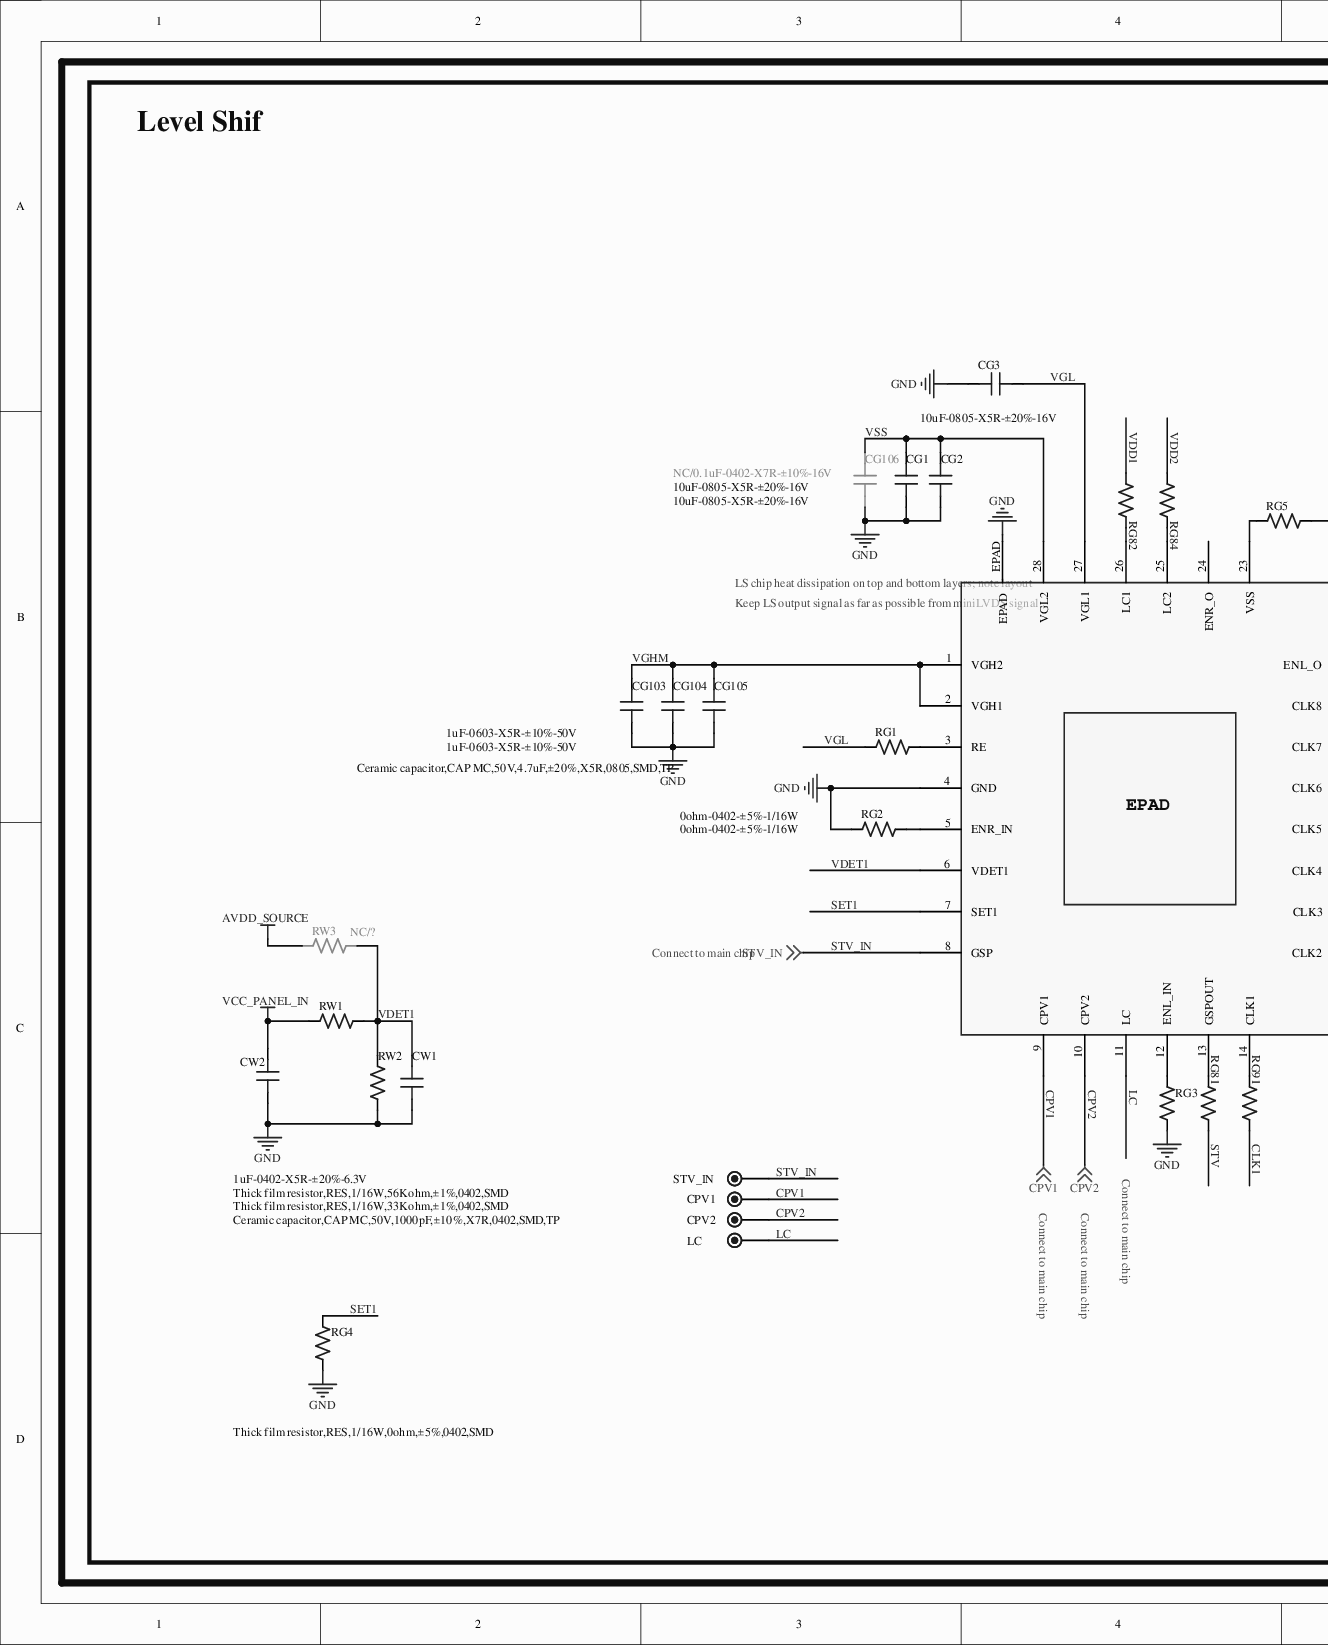
[diagram p0: MISC84395-19.SchDoc, left]
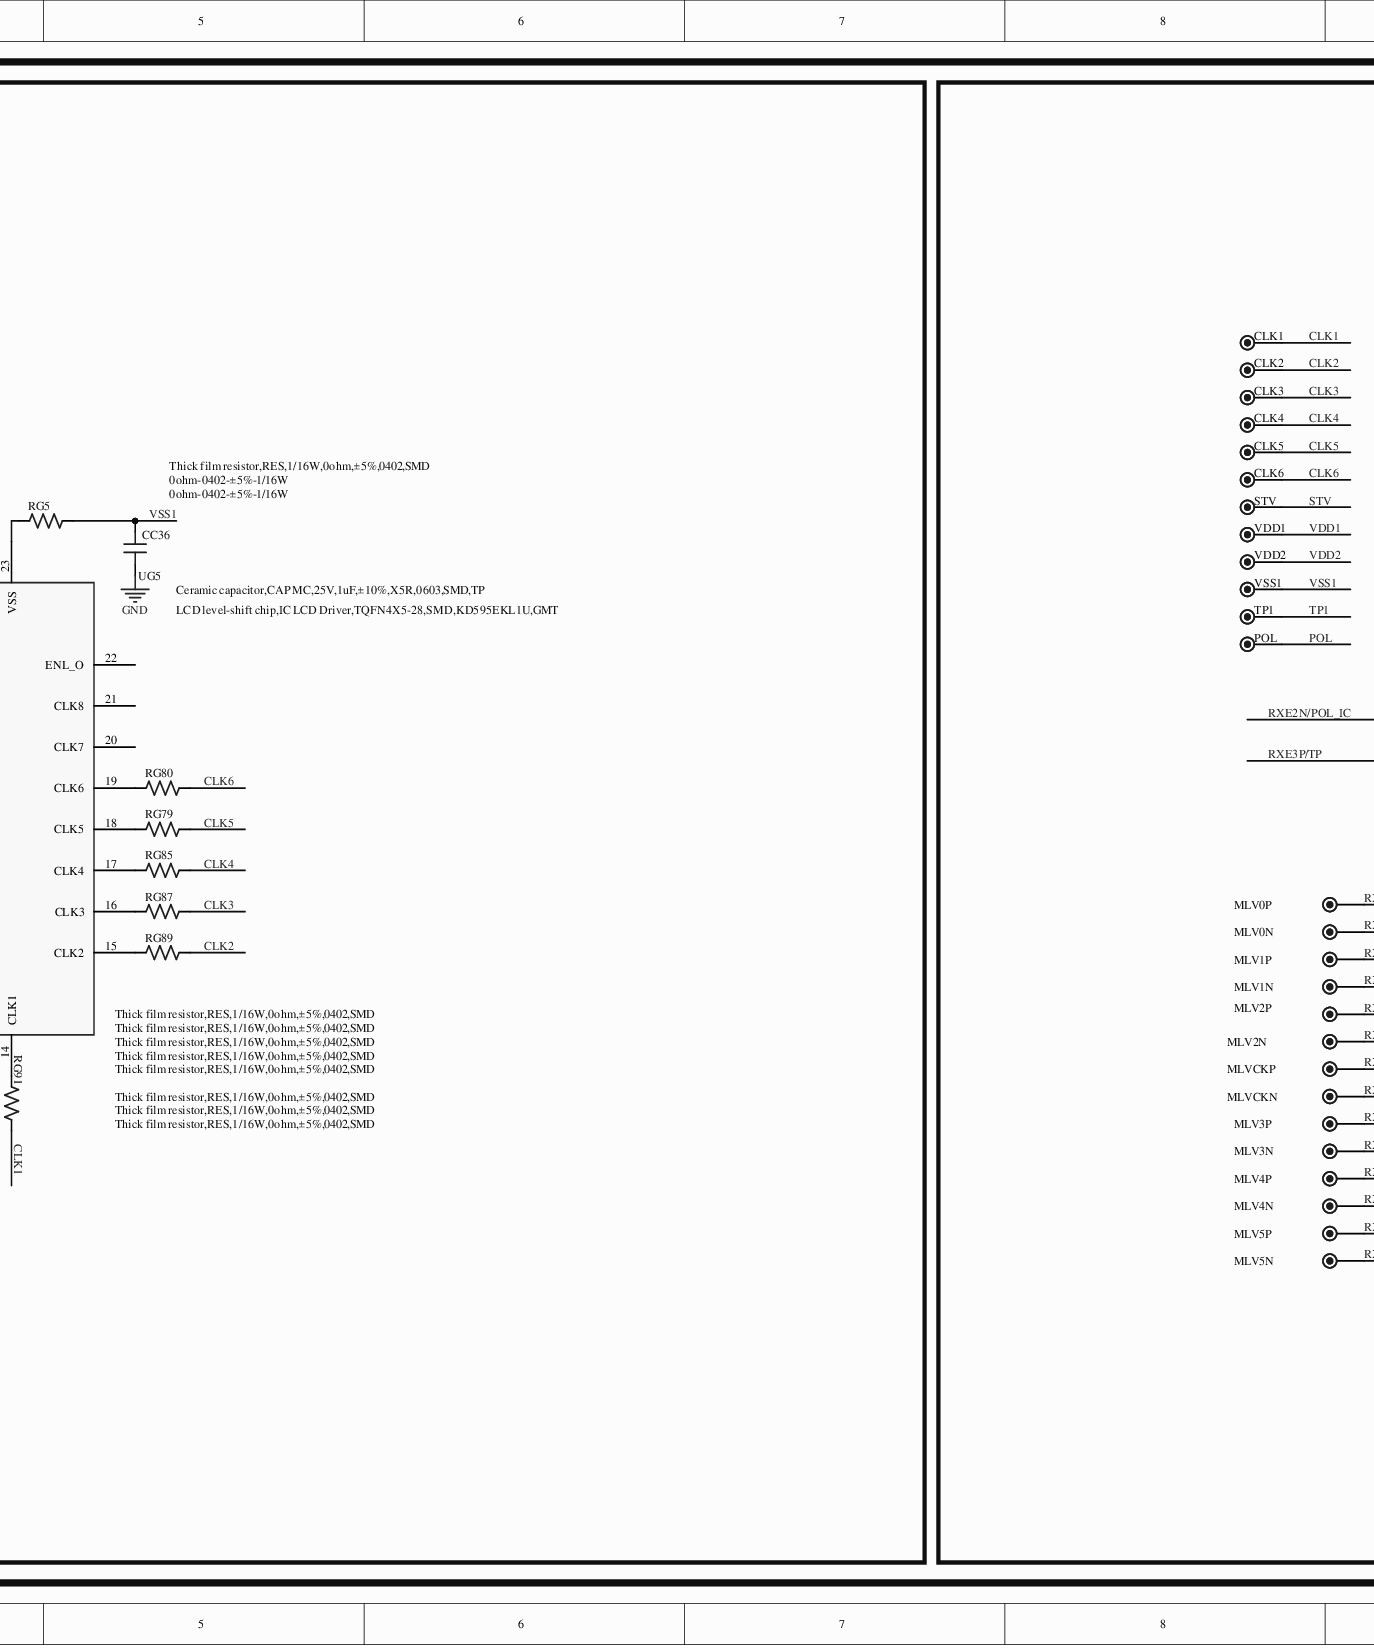
[diagram p1: MISC84395-19.SchDoc, middle]
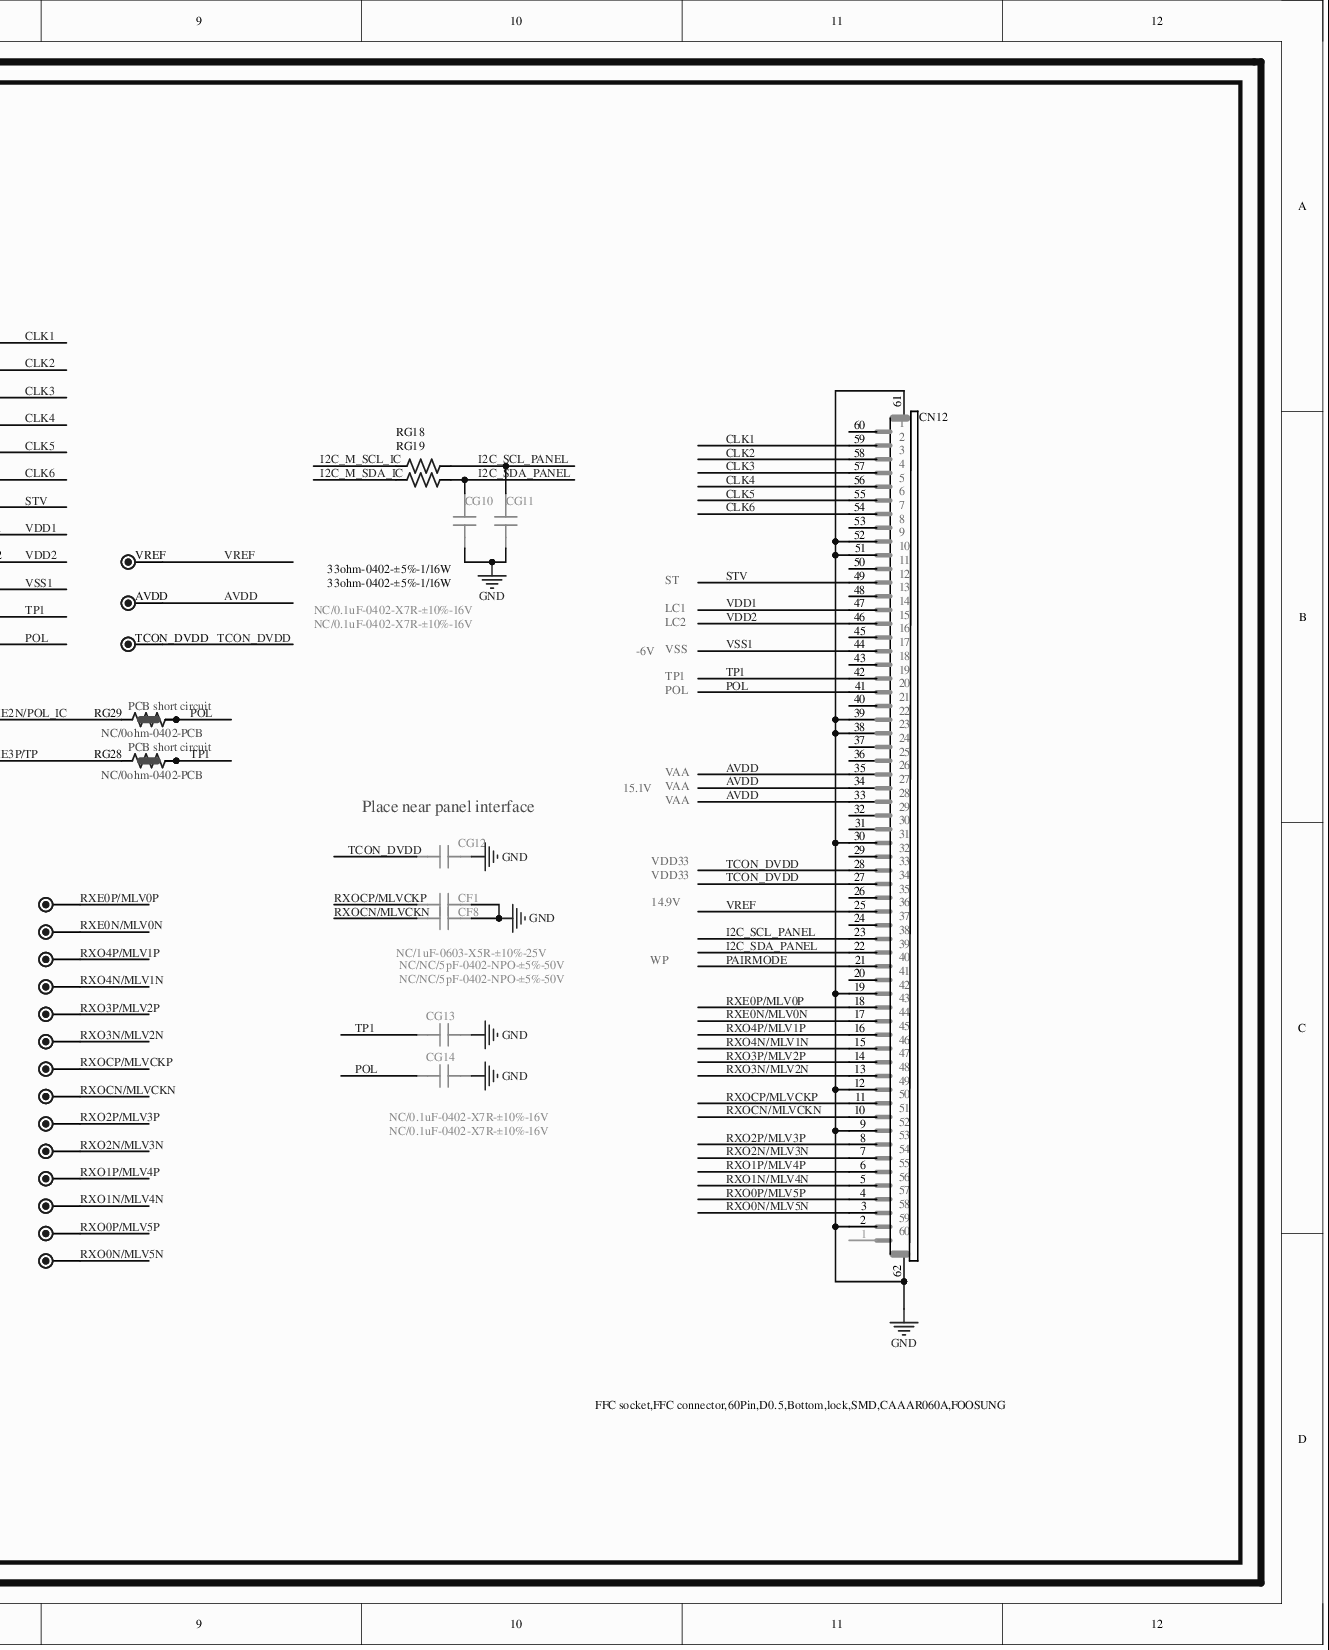
[diagram p2: MISC84395-19.SchDoc, right]
# Altium project MISC84395-37.PrjPCB (part 13 of 13)

## Sheet MISC84395-19.SchDoc
size 711 x 304 mm

### Parts
AVDD  TEST  [TP]  (value not drawn)
CC36  Ceramic capacitor,CAP MC,25V,1uF,±10%,X5R,0603,SMD,TP  [C0603]
CF1  NC/NC/5pF-0402-NPO-±5%-50V  [C0402]
CF8  NC/NC/5pF-0402-NPO-±5%-50V  [C0402]
CG1  10uF-0805-X5R-±20%-16V  [C0805]
CG2  10uF-0805-X5R-±20%-16V  [C0805]
CG3  10uF-0805-X5R-±20%-16V  [C0805]
CG10  NC/0.1uF-0402-X7R-±10%-16V  [C0402]
CG11  NC/0.1uF-0402-X7R-±10%-16V  [C0402]
CG12  NC/1uF-0603-X5R-±10%-25V  [C0603]
CG13  NC/0.1uF-0402-X7R-±10%-16V  [C0402]
CG14  NC/0.1uF-0402-X7R-±10%-16V  [C0402]
CG103  1uF-0603-X5R-±10%-50V  [C0603]
CG104  Ceramic capacitor,CAP MC,50V,4.7uF,±20%,X5R,0805,SMD,TP  [C0805]
CG105  1uF-0603-X5R-±10%-50V  [C0603]
CG106  NC/0.1uF-0402-X7R-±10%-16V  [C0402]
CLK1  TEST  [TP]  (value not drawn)
CLK2  TEST  [TP]  (value not drawn)
CLK3  TEST  [TP]  (value not drawn)
CLK4  TEST  [TP]  (value not drawn)
CLK5  TEST  [TP]  (value not drawn)
CLK6  TEST  [TP]  (value not drawn)
CN12  FFC socket,FFC connector,60Pin,D0.5,Bottom,lock,SMD,CAAAR060A,FOOSUNG  [FFC60H/0.5S-13]
CPV1  TEST  [TP]  (value not drawn)
CPV2  TEST  [TP]  (value not drawn)
CW1  Ceramic capacitor,CAP MC,50V,1000pF,±10%,X7R,0402,SMD,TP  [C0402]
CW2  1uF-0402-X5R-±20%-6.3V  [C0402]
LC  TEST  [TP]  (value not drawn)
MLV0N  TEST  [TP]  (value not drawn)
MLV0P  TEST  [TP]  (value not drawn)
MLV1N  TEST  [TP]  (value not drawn)
MLV1P  TEST  [TP]  (value not drawn)
MLV2N  TEST  [TP]  (value not drawn)
MLV2P  TEST  [TP]  (value not drawn)
MLV3N  TEST  [TP]  (value not drawn)
MLV3P  TEST  [TP]  (value not drawn)
MLV4N  TEST  [TP]  (value not drawn)
MLV4P  TEST  [TP]  (value not drawn)
MLV5N  TEST  [TP]  (value not drawn)
MLV5P  TEST  [TP]  (value not drawn)
MLVCKN  TEST  [TP]  (value not drawn)
MLVCKP  TEST  [TP]  (value not drawn)
POL  TEST  [TP]  (value not drawn)
RG1  0ohm-0402-±5%-1/16W  [R0402]
RG2  0ohm-0402-±5%-1/16W  [R0402]
RG3  Thick film resistor,RES,1/16W,0ohm,±5%,0402,SMD  [R0402]
RG4  Thick film resistor,RES,1/16W,0ohm,±5%,0402,SMD  [R0402]
RG5  0ohm-0402-±5%-1/16W  [R0402]
RG18  33ohm-0402-±5%-1/16W  [R0402]
RG19  33ohm-0402-±5%-1/16W  [R0402]
RG28  NC/0ohm-0402-PCB  [R0402SC]
RG29  NC/0ohm-0402-PCB  [R0402SC]
RG79  Thick film resistor,RES,1/16W,0ohm,±5%,0402,SMD  [R0402]
RG80  Thick film resistor,RES,1/16W,0ohm,±5%,0402,SMD  [R0402]
RG81  Thick film resistor,RES,1/16W,0ohm,±5%,0402,SMD  [R0402]
RG82  Thick film resistor,RES,1/16W,0ohm,±5%,0402,SMD  [R0402]
RG84  0ohm-0402-±5%-1/16W  [R0402]
RG85  Thick film resistor,RES,1/16W,0ohm,±5%,0402,SMD  [R0402]
RG87  Thick film resistor,RES,1/16W,0ohm,±5%,0402,SMD  [R0402]
RG89  Thick film resistor,RES,1/16W,0ohm,±5%,0402,SMD  [R0402]
RG91  Thick film resistor,RES,1/16W,0ohm,±5%,0402,SMD  [R0402]
RW1  Thick film resistor,RES,1/16W,56Kohm,±1%,0402,SMD  [R0402]
RW2  Thick film resistor,RES,1/16W,33Kohm,±1%,0402,SMD  [R0402]
RW3  NC/?  [R0402]
STV  TEST  [TP]  (value not drawn)
STV_IN  TEST  [TP]  (value not drawn)
TCON_DVDD  TEST  [TP]  (value not drawn)
TP1  TEST  [TP]  (value not drawn)
UG5  LCD level-shift chip,IC LCD Driver,TQFN4X5-28,SMD,KD595EKL1U,GMT  [QFN28/0.5-5]
VDD1  TEST  [TP]  (value not drawn)
VDD2  TEST  [TP]  (value not drawn)
VREF  TEST  [TP]  (value not drawn)
VSS1  TEST  [TP]  (value not drawn)

### Blocks framed on the sheet
Level Shif: CC36 CG1-CG3 CG103-CG106 CPV1 CPV2 CW1 CW2 LC RG1-RG5 RG79-RG82 RG84 RG85 RG87 RG89 RG91 RW1-RW3 STV_IN UG5
Place near panel interface: AVDD CF1 CF8 CG10-CG14 CLK1-CLK6 CN12 MLV0N MLV0P MLV1N MLV1P MLV2N MLV2P MLV3N MLV3P MLV4N MLV4P MLV5N MLV5P MLVCKN MLVCKP POL RG18 RG19 RG28 RG29 STV TCON_DVDD TP1 VDD1 VDD2 VREF VSS1

### Nets
AVDD: AVDD.1 CN12.33 CN12.34 CN12.35
AVDD_SOURCE: RW3.1
GND: CC36.2 CF1.1 CF8.1 CG1.2 CG2.2 CG3.2 CG10.1 CG11.1 CG12.1 CG13.1 CG14.1 CG103.1 CG104.2 CG105.1 CG106.1 CN12.2 CN12.9 CN12.12 CN12.19 CN12.30 CN12.38 CN12.39 CN12.51 CN12.52 CN12.61 CN12.62 CW1.1 CW2.2 RG2.1 RG3.1 RG4.1 RW2.1 UG5.4(GND) UG5.EPAD
TCON_DVDD: CG12.2 CN12.27 CN12.28 TCON_DVDD.1
VCC_PANEL_IN: CW2.1 RW1.1
VGL: CG3.1 RG1.1 UG5.27(VGL1)
VREF: CN12.25 VREF.1
CLK1: CLK1.1 CN12.59 RG91.2
CLK2: CLK2.1 CN12.58 RG89.2
CLK3: CLK3.1 CN12.57 RG87.2
CLK4: CLK4.1 CN12.56 RG85.2
CLK5: CLK5.1 CN12.55 RG79.1
CLK6: CLK6.1 CN12.54 RG80.1
CPV1: CPV1.1 UG5.9(CPV1) ; off-sheet CPV1
CPV2: CPV2.1 UG5.10(CPV2) ; off-sheet CPV2
I2C_M_SCL_IC: RG18.1
I2C_M_SDA_IC: RG19.1
I2C_SCL_PANEL: CG11.2 CN12.23 RG18.2
I2C_SDA_PANEL: CG10.2 CN12.22 RG19.2
LC: LC.1 UG5.11(LC)
PAIRMODE: CN12.21
POL: CG14.2 CN12.41 POL.1 RG29.2 RG29.3
RXE0N/MLV0N: CN12.17 MLV0N.1
RXE0P/MLV0P: CN12.18 MLV0P.1
RXE2N/POL_IC: RG29.1
RXE3P/TP: RG28.1
RXO0N/MLV5N: CN12.3 MLV5N.1
RXO0P/MLV5P: CN12.4 MLV5P.1
RXO1N/MLV4N: CN12.5 MLV4N.1
RXO1P/MLV4P: CN12.6 MLV4P.1
RXO2N/MLV3N: CN12.7 MLV3N.1
RXO2P/MLV3P: CN12.8 MLV3P.1
RXO3N/MLV2N: CN12.13 MLV2N.1
RXO3P/MLV2P: CN12.14 MLV2P.1
RXO4N/MLV1N: CN12.15 MLV1N.1
RXO4P/MLV1P: CN12.16 MLV1P.1
RXOCN/MLVCKN: CF8.2 CN12.10 MLVCKN.1
RXOCP/MLVCKP: CF1.2 CN12.11 MLVCKP.1
SET1: RG4.2 UG5.7(SET1)
STV: CN12.49 RG81.1 STV.1
STV_IN: STV_IN.1 UG5.8(GSP) ; off-sheet STV_IN
TP1: CG13.2 CN12.42 RG28.2 RG28.3 TP1.1
VDD1: CN12.47 RG82.1 VDD1.1
VDD2: CN12.46 RG84.1 VDD2.1
VDET1: CW1.2 RW1.2 RW2.2 RW3.2 UG5.6(VDET1)
VGHM: CG103.2 CG104.1 CG105.2 UG5.1(VGH2) UG5.2(VGH1)
VSS: CG1.1 CG2.1 CG106.2 UG5.28(VGL2)
VSS1: CC36.1 CN12.44 RG5.1 VSS1.1
NetRG1_2: RG1.2 UG5.3(RE)
NetRG2_2: RG2.2 UG5.5(ENR_IN)
NetRG3_2: RG3.2 UG5.12(ENL_IN)
NetRG5_2: RG5.2 UG5.23(VSS)
NetRG79_2: RG79.2 UG5.18(CLK5)
NetRG80_2: RG80.2 UG5.19(CLK6)
NetRG81_2: RG81.2 UG5.13(GSPOUT)
NetRG82_2: RG82.2 UG5.26(LC1)
NetRG84_2: RG84.2 UG5.25(LC2)
NetRG85_1: RG85.1 UG5.17(CLK4)
NetRG87_1: RG87.1 UG5.16(CLK3)
NetRG89_1: RG89.1 UG5.15(CLK2)
NetRG91_1: RG91.1 UG5.14(CLK1)

Not connected (* = marked no-connect by the designer): CN12 1* 20* 24* 26* 29* 31* 32* 36* 37* 40* 43* 45* 48* 50* 53* 60*; UG5 20(CLK7)* 21(CLK8)* 22(ENL_O)* 24(ENR_O)*

### Notes on the sheet
- (near CN12) 1
- (near CN12) 2
- (near CN12) 3
- (near CN12) 4
- (near CN12) 5
- (near CN12) 6
- (near CN12) 7
- (near CN12) 8
- (near CN12) 9
- (near CN12) 10
- (near CN12) 11
- (near CN12) 12
- (near UG5) LS chip heat dissipation on top and bottom layers; note layout
- (near UG5) Keep LS output signal as far as possible from miniLVDS signal
- LC1
- LC2
- ST
- (near CN12) 13
- (near CN12) 14
- (near CN12) 15
- (near CN12) 16
- (near CN12) 17
- -6V
- VSS
- TP1
- POL
- (near CN12) 18
- (near CN12) 19
- (near CN12) 20
- (near CN12) 21
- (near CN12) 22
- VAA
- (near CN12) 23
- (near CN12) 24
- (near CN12) 25
- (near CN12) 26
- (near CN12) 27
- 15.1V
- (near CN12) 28
- (near CN12) 29
- (near CN12) 30
- (near CN12) 31
- (near CN12) 32
- VDD33
- 14.9V
- (near CN12) 33
- (near CN12) 34
- (near CN12) 35
- (near CN12) 36
- (near CN12) 37
- Connect to main chip
- WP
- (near CN12) 38
- (near CN12) 39
- (near CN12) 40
- (near CN12) 41
- (near CN12) 42
- (near CN12) 43
- (near CN12) 44
- (near CN12) 45
- (near CN12) 46
- (near CN12) 47
- (near CN12) 48
- (near CN12) 49
- (near CN12) 50
- (near CN12) 51
- (near CN12) 52
- (near CN12) 53
- (near CN12) 54
- (near CN12) 55
- (near CN12) 56
- (near CN12) 57
- (near CN12) 58
- (near CN12) 59
- (near CN12) 60

### Library data of the parts
CC36 CG12 CG103 CG105 = 1uF-0603-X5R-±10%-50V-D
CF1 CF8 = 5pF-0402-NPO-±5%-50V-D
CG1-CG3 CG104 = 10uF-0805-X5R-±20%-16V-D
CG10 CG11 CG13 CG14 CG106 CW2 = 0.1uF-0402-X5R-±20%-16V-D
CN12 = XXX.XXX.0004785-D: FFC socket,FFC connector,60Pin,D0.5,Bottom,lock,SMD,CAAAR060A,FOOSUNG-D
CW1 = 004.003.0000503-D: Ceramic capacitor,CAP MC,50V,1000pF,±10%,X7R,0402,SMD,TP-D
RG1-RG5 RG79-RG82 RG84 RG85 RG87 RG89 RG91 = 22ohm-0402-±5%-1/16W-D
RG18 RG19 = 33ohm-0402-±5%-1/16W-D
RG28 RG29 = 0ohm-0402-PCB-D
RW1 RW3 = 004.002.0000488-D: Thick film resistor,RES,1/16W,56Kohm,±1%,0402,SMD-D
RW2 = 004.002.0000104-D: Thick film resistor,RES,1/16W,33Kohm,±1%,0402,SMD-D
UG5 = 004.022.0000213-D: LCD level-shift chip,IC Driver,TQFN4X5-28,SMD,G2595EKL1U-K,GMT-D

## Nets that join several sheets
1V8_M: MISC84395-7 (5 pins), MISC84395-9 (R45.1), MISC84395-11 (R4.1)
3V3_M: MISC84395-7 (5 pins), MISC84395-8 (RT34.2 RT36.2 RT39.2 RT40.2), MISC84395-9 (11 pins), MISC84395-11 (9 pins), MISC84395-14 (RU3.2 RU9.2), MISC84395-17 (CT14.1 LT20.1 RT7.1), MISC84395-18 (LG02.2)
3V3_STB: MISC84395-7 (11 pins), MISC84395-8 (C103.2 R30.1 R34.1 U6.3), MISC84395-9 (13 pins), MISC84395-15 (RK1.2 RM13.2)
5V_M: MISC84395-7 (9 pins), MISC84395-12 (RI1.1), MISC84395-14 (CU.1 U16.5), MISC84395-15 (R12.1), MISC84395-17 (CT3.2 CT4.1 UTL1.3), MISC84395-18 (RG02.2)
5V_STB: MISC84395-7 (19 pins), MISC84395-8 (RV15.2 RV17.2), MISC84395-15 (5 pins)
12V: MISC84395-7 (16 pins), MISC84395-8 (R27.2), MISC84395-16 (13 pins), MISC84395-4 (15 pins)
+1.5V_DDR: MISC84395-7 (7 pins), MISC84395-9 (21 pins), MISC84395-10 (40 pins)
+1.05V_VDDC_CPU: MISC84395-7 (9 pins), MISC84395-9 (18 pins)
+1.10V_VDDC: MISC84395-7 (10 pins), MISC84395-9 (26 pins)
ADIM: MISC84395-7 (CL13.2 QL1.C RL1.2 RL12.1), MISC84395-4 (ADIM.1 RB833.2)
AVDD: MISC84395-18 (15 pins), MISC84395-19 (AVDD.1 CN12.33 CN12.34 CN12.35)
AVDD_SOURCE: MISC84395-7 (CM13.1 QM8.D), MISC84395-18 (CC8.1 CC12.1 CC13.2 LC1.1), MISC84395-19 (RW3.1)
BL_ON: MISC84395-7 (CL10.2 RL6.1), MISC84395-4 (BL_ON.1 RB802.1)
GND: MISC84395-3 (24 pins), MISC84395-5 (6 pins), MISC84395-7 (76 pins), MISC84395-8 (23 pins), MISC84395-9 (164 pins), MISC84395-10 (82 pins), MISC84395-11 (28 pins), MISC84395-12 (21 pins), MISC84395-13 (36 pins), MISC84395-14 (26 pins), MISC84395-15 (19 pins), MISC84395-16 (27 pins), MISC84395-17 (59 pins), MISC84395-18 (59 pins), MISC84395-4 (46 pins), MISC84395-19 (34 pins)
PWM_DIM: MISC84395-7 (CL14.2 QL2.C RL2.1 RL5.1), MISC84395-4 (PWM_DIM.1 RB801.1)
TCON_DVDD: MISC84395-18 (8 pins), MISC84395-19 (CG12.2 CN12.27 CN12.28 TCON_DVDD.1)
VCC_PANEL_IN: MISC84395-7 (7 pins), MISC84395-18 (6 pins), MISC84395-19 (CW2.1 RW1.1)
VGL: MISC84395-18 (9 pins), MISC84395-19 (CG3.1 RG1.1 UG5.27)
VREF: MISC84395-18 (8 pins), MISC84395-19 (CN12.25 VREF.1)
AMP_L_OUT_IC: MISC84395-8 (U5.W3), MISC84395-16 (DA2.K RA13.1)
AMP_MUTE_IC: MISC84395-8 (U5.H18), MISC84395-16 (RA31.2 RA32.2)
AMP_R_OUT_IC: MISC84395-8 (U5.Y3), MISC84395-16 (DA1.K RA6.1)
AV/YPbPr_L_IN_IC: MISC84395-8 (U5.Y2), MISC84395-12 (CI6.2)
AV/YPbPr_R_IN_IC: MISC84395-8 (U5.W1), MISC84395-12 (CI9.2)
AV_CVBS_IN_IC: MISC84395-8 (U5.T4), MISC84395-12 (CI4.1)
BL_DIM_OUT_IC: MISC84395-7 (RL4.1 RL5.2 RL9.2 RL11.1), MISC84395-8 (U5.V18)
BL_ON_IC: MISC84395-7 (CL15.2 RL6.2 RL8.2), MISC84395-8 (U5.L4)
BT_RESET: MISC84395-8 (R1.1), MISC84395-15 (BT_RST.1 CN1.9 CU5.2)
CPV1: MISC84395-8 (U5.AA19), MISC84395-19 (CPV1.1 UG5.9)
CPV2: MISC84395-8 (U5.AA18), MISC84395-19 (CPV2.1 UG5.10)
DCDC_SCL_IC: MISC84395-7 (RD19.2), MISC84395-8 (D11.K RT34.1 U5.E5)
DCDC_SDA_IC: MISC84395-7 (RD18.2), MISC84395-8 (D12.K RT36.1 U5.E4)
DDR_EN_IC: MISC84395-7 (RD3.2), MISC84395-8 (R30.2 U5.K5)
EMMC_CLK_IC: MISC84395-8 (U5.W12), MISC84395-11 (R5.2)
EMMC_CMD_IC: MISC84395-8 (U5.AA13), MISC84395-11 (5 pins)
EMMC_D0_IC: MISC84395-8 (U5.AA9), MISC84395-11 (RP2.8)
EMMC_D1_IC: MISC84395-8 (U5.W9), MISC84395-11 (RP1.2)
EMMC_D2_IC: MISC84395-8 (U5.AA10), MISC84395-11 (RP1.4)
EMMC_D3_IC: MISC84395-8 (U5.Y9), MISC84395-11 (RP2.6)
EMMC_D4_IC: MISC84395-8 (U5.W8), MISC84395-11 (RP2.4)
EMMC_D5_IC: MISC84395-8 (U5.Y8), MISC84395-11 (RP2.2)
EMMC_D6_IC: MISC84395-8 (U5.W10), MISC84395-11 (RP1.8)
EMMC_D7_IC: MISC84395-8 (U5.Y10), MISC84395-11 (RP1.6)
EMMC_DS_IC: MISC84395-8 (U5.W11), MISC84395-11 (R11.2 U1.H5)
EMMC_RST_IC: MISC84395-8 (U5.Y12), MISC84395-11 (5 pins)
HDMI1_CLKN_IC: MISC84395-8 (U5.J1), MISC84395-13 (AVH1.12 UH8.4 UH8.5)
HDMI1_CLKP_IC: MISC84395-8 (U5.J2), MISC84395-13 (AVH1.10 UH8.3 UH8.6)
HDMI1_DET_IC: MISC84395-8 (U5.R4), MISC84395-13 (RH8.2)
HDMI1_HPD_IC: MISC84395-8 (U5.R5), MISC84395-13 (RH2.2 RH3.2)
HDMI1_RX0N_IC: MISC84395-8 (U5.K3), MISC84395-13 (AVH1.9 UH8.2 UH8.7)
HDMI1_RX0P_IC: MISC84395-8 (U5.K2), MISC84395-13 (AVH1.7 UH8.1 UH8.8)
HDMI1_RX1N_IC: MISC84395-8 (U5.L3), MISC84395-13 (AVH1.6 UH7.4 UH7.5)
HDMI1_RX1P_IC: MISC84395-8 (U5.L2), MISC84395-13 (AVH1.4 UH7.3 UH7.6)
HDMI1_RX2N_IC: MISC84395-8 (U5.L1), MISC84395-13 (AVH1.3 UH7.2 UH7.7)
HDMI1_RX2P_IC: MISC84395-8 (U5.M2), MISC84395-13 (AVH1.1 UH7.1 UH7.8)
HDMI1_SCL_IC: MISC84395-8 (U5.P6), MISC84395-13 (RH7.2)
HDMI1_SDA_IC: MISC84395-8 (U5.R6), MISC84395-13 (RH6.2)
HDMI2_CLKN_IC: MISC84395-8 (U5.F3), MISC84395-13 (AVH2.12 UH6.4 UH6.5)
HDMI2_CLKP_IC: MISC84395-8 (U5.F1), MISC84395-13 (AVH2.10 UH6.3 UH6.6)
HDMI2_DET_IC: MISC84395-8 (U5.P5), MISC84395-13 (RH18.2)
HDMI2_HPD_IC: MISC84395-8 (U5.P4), MISC84395-13 (RH11.2 RH12.2)
HDMI2_RX0N_IC: MISC84395-8 (U5.F2), MISC84395-13 (AVH2.9 UH6.2 UH6.7)
HDMI2_RX0P_IC: MISC84395-8 (U5.G3), MISC84395-13 (AVH2.7 UH6.1 UH6.8)
HDMI2_RX1N_IC: MISC84395-8 (U5.G2), MISC84395-13 (AVH2.6 UH5.4 UH5.5)
HDMI2_RX1P_IC: MISC84395-8 (U5.H3), MISC84395-13 (AVH2.4 UH5.3 UH5.6)
HDMI2_RX2N_IC: MISC84395-8 (U5.H2), MISC84395-13 (AVH2.3 UH5.2 UH5.7)
HDMI2_RX2P_IC: MISC84395-8 (U5.H1), MISC84395-13 (AVH2.1 UH5.1 UH5.8)
HDMI2_SCL_IC: MISC84395-8 (U5.N5), MISC84395-13 (RH17.2)
HDMI2_SDA_IC: MISC84395-8 (U5.N4), MISC84395-13 (RH16.2)
HDMI_ARC_IC: MISC84395-8 (U5.N6), MISC84395-13 (CH2.2)
HDMI_CEC_IC: MISC84395-8 (U5.N3), MISC84395-13 (RH13.2)
I2C_M_SCL_IC: MISC84395-8 (D13.K RT39.1 U5.AA7), MISC84395-17 (RT10.1), MISC84395-19 (RG18.1)
I2C_M_SDA_IC: MISC84395-8 (D14.K RT40.1 U5.W6), MISC84395-17 (RT5.1), MISC84395-19 (RG19.1)
IR_IN_IC: MISC84395-8 (U5.V5), MISC84395-15 (RK14.2)
KEY0_IN_IC: MISC84395-8 (U5.C5), MISC84395-15 (CK2.1 RK2.1)
LC: MISC84395-8 (U5.Y17), MISC84395-19 (LC.1 UG5.11)
LED_R: MISC84395-8 (R37.2 U5.L5), MISC84395-15 (RK8.1)
LED_R_OFF: MISC84395-8 (R34.2 U5.U3), MISC84395-15 (RK4.1)
NX_ADJ_IC: MISC84395-7 (RL1.1 RL3.1 RL7.2 RL10.1), MISC84395-8 (U5.U17)
PAIRMODE: MISC84395-18 (RG17.2 RG24.2 RG30.1), MISC84395-19 (CN12.21)
PAIRMODE/: MISC84395-8 (U5.J18), MISC84395-18 (RG17.1)
PANEL_EN_IC: MISC84395-7 (RM8.1), MISC84395-8 (U5.B4)
PHY_RX_N_IC: MISC84395-8 (U5.C4), MISC84395-14 (RE14.1)
PHY_RX_P_IC: MISC84395-8 (U5.B3), MISC84395-14 (RE13.1)
PHY_TX_N_IC: MISC84395-8 (U5.A3), MISC84395-14 (RE12.1)
PHY_TX_P_IC: MISC84395-8 (U5.A2), MISC84395-14 (RE11.1)
PWR_ON/OFF_IC: MISC84395-7 (RM4.2 RM7.1), MISC84395-8 (U5.K4)
RXE0N/MLV0N: MISC84395-8 (U5.M20), MISC84395-19 (CN12.17 MLV0N.1)
RXE0P/MLV0P: MISC84395-8 (U5.L19), MISC84395-19 (CN12.18 MLV0P.1)
RXE2N/POL_IC: MISC84395-8 (U5.Y20), MISC84395-19 (RG29.1)
RXE3P/TP: MISC84395-8 (U5.Y18), MISC84395-19 (RG28.1)
RXO0N/MLV5N: MISC84395-8 (U5.V21), MISC84395-19 (CN12.3 MLV5N.1)
RXO0P/MLV5P: MISC84395-8 (U5.V20), MISC84395-19 (CN12.4 MLV5P.1)
RXO1N/MLV4N: MISC84395-8 (U5.U20), MISC84395-19 (CN12.5 MLV4N.1)
RXO1P/MLV4P: MISC84395-8 (U5.T19), MISC84395-19 (CN12.6 MLV4P.1)
RXO2N/MLV3N: MISC84395-8 (U5.T21), MISC84395-19 (CN12.7 MLV3N.1)
RXO2P/MLV3P: MISC84395-8 (U5.R19), MISC84395-19 (CN12.8 MLV3P.1)
RXO3N/MLV2N: MISC84395-8 (U5.N19), MISC84395-19 (CN12.13 MLV2N.1)
RXO3P/MLV2P: MISC84395-8 (U5.N20), MISC84395-19 (CN12.14 MLV2P.1)
RXO4N/MLV1N: MISC84395-8 (U5.M19), MISC84395-19 (CN12.15 MLV1N.1)
RXO4P/MLV1P: MISC84395-8 (U5.M21), MISC84395-19 (CN12.16 MLV1P.1)
RXOCN/MLVCKN: MISC84395-8 (U5.R20), MISC84395-19 (CF8.2 CN12.10 MLVCKN.1)
RXOCP/MLVCKP: MISC84395-8 (U5.P19), MISC84395-19 (CF1.2 CN12.11 MLVCKP.1)
SPDIF_OUT_IC: MISC84395-8 (U5.F5), MISC84395-12 (CO19.2 DO1.K RO45.1)
STV_IN: MISC84395-8 (U5.W19), MISC84395-19 (STV_IN.1 UG5.8)
Tun_AGC_IN_IC: MISC84395-8 (U5.Y7), MISC84395-17 (CT13.2 RT7.2 RT9.2)
Tun_IFM_OUT_IC: MISC84395-8 (U5.Y6), MISC84395-17 (CT9.2)
Tun_IFP_OUT_IC: MISC84395-8 (U5.AA6), MISC84395-17 (CT2.2)
USB2_DM_IC: MISC84395-8 (U5.A6), MISC84395-15 (RU1.2 RU1.3)
USB2_DP_IC: MISC84395-8 (U5.C6), MISC84395-15 (RU6.2 RU6.3)
USB3_DM_IC: MISC84395-8 (U5.A5), MISC84395-14 (DU1.K RU4.2 RU4.3)
USB3_DP_IC: MISC84395-8 (U5.B5), MISC84395-14 (DU2.K RU5.2 RU5.3)
USB_EN_IC: MISC84395-8 (U5.H4), MISC84395-14 (DU9.K RU12.1)
USB_FLT_IC: MISC84395-8 (U5.G4), MISC84395-14 (DU8.K RU7.1)
VGHM: MISC84395-18 (CC14.2 RC5.1 RG6.2), MISC84395-19 (5 pins)
VID0_OUT_IC: MISC84395-7 (RD24.2 RD40.1), MISC84395-8 (U5.G5)
VSS: MISC84395-18 (CC43.2 RC36.2), MISC84395-19 (CG1.1 CG2.1 CG106.2 UG5.28)
WIFI_RESET: MISC84395-8 (R2.1), MISC84395-15 (CN1.8 CU4.2 WIFI_RST.1)